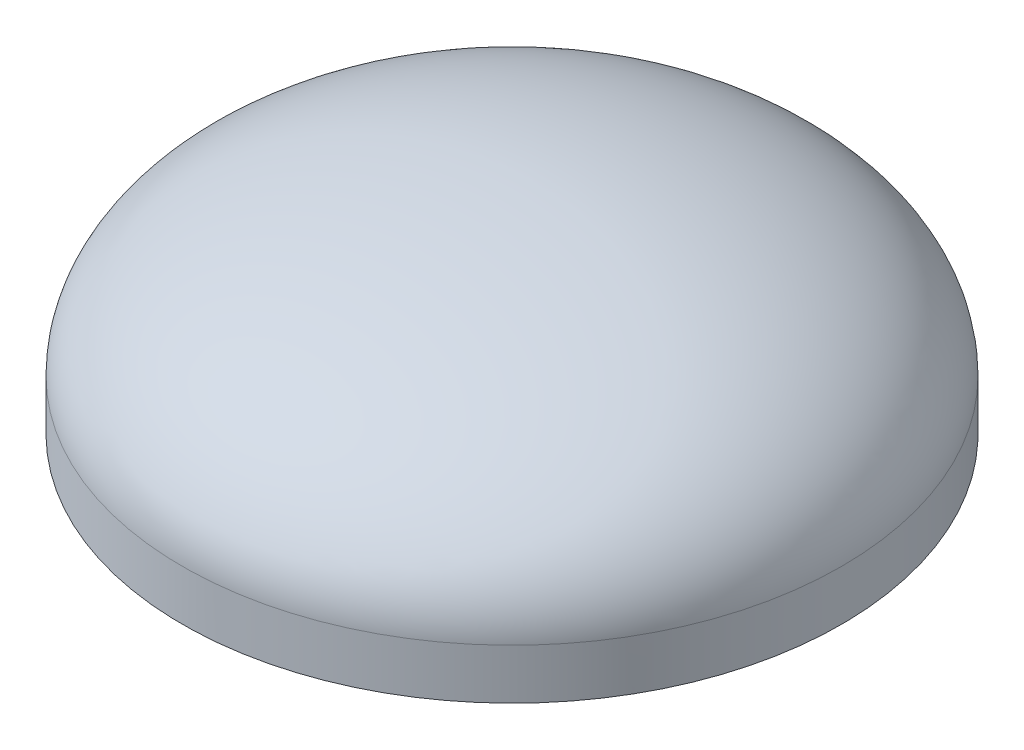
SolidWorks part; units mm, degrees
material "Plain carbon steel"
ref_plane "Front Plane" through (0, 0, 0) normal (0, 0, 1) x (1, 0, 0)
ref_plane "Top Plane" through (0, 0, 0) normal (0, 1, 0) x (1, 0, 0)
ref_plane "Right Plane" through (0, 0, 0) normal (1, 0, 0) x (0, 0, -1)
sketch "Sketch1" plane through (0, 0, 0) normal (0, 0, 1) x (1, 0, 0)
  line L0 (0, 0) -> (162.5, 0) construction
  line L1 (0, 0) -> (0, 106) construction
  point P3 (162.5, 0)
  point P6 (0, 6)
  dimension "DN" = 325
  dimension "H" = 106
  dimension "δ" = 6
sketch "Sketch2" plane through (0, 0, 0) normal (0, 0, 1) x (1, 0, 0)
  line L0 (-162.5, 0) -> (162.5, 0) construction
  line L1 (0, 0) -> (162.5, 0) construction
  line L3 (0, 0) -> (0, 81.25) construction
  line L4 (0, 0) -> (0, -24.75) construction
  line L5 (-162.5, 0) -> (-168.5, 0) construction
  line L6 (0, 81.25) -> (0, 87.25) construction
  line L7 (162.5, 0) -> (168.5, 0) construction
  line L8 (-168.5, 0) -> (-168.5, -24.75)
  line L9 (-168.5, -24.75) -> (-162.5, -24.75)
  line L10 (-162.5, -24.75) -> (-162.5, 0)
  line L11 (0, 81.25) -> (0, 87.25)
  ellipse E0 centre (0, 0) end of major axis (162.5, 0) minor radius 81.25 (0, 81.25) -> (-162.5, 0) ccw
  ellipse E1 centre (0, 0) end of major axis (168.5, 0) minor radius 87.25 (0, 87.25) -> (-168.5, 0) ccw
  dimension "Di" = 325
  dimension "h" = 24.75
  dimension "(H)" = 106
  dimension "δ" = 6
revolve "Revolve1" [suppressed] add sketch "Sketch2" angle 360 mid plane about L3
sketch "Sketch3" plane through (0, 0, 0) normal (0, 0, 1) x (1, 0, 0)
  line L0 (0, 0) -> (0, 81.25) construction
  line L1 (-162.5, 0) -> (162.5, 0) construction
  line L2 (0, 0) -> (162.5, 0) construction
  line L3 (-162.5, -24.75) -> (162.5, -24.75) construction
  line L4 (-162.5, 0) -> (-162.5, -24.75)
  line L5 (-162.5, -24.75) -> (-159.5, -24.75)
  line L6 (-159.5, -24.75) -> (-159.5, 0)
  line L7 (0, 81.25) -> (0, 78.25)
  ellipse E0 centre (0, 0) end of major axis (162.5, 0) minor radius 81.25 (0, 81.25) -> (-162.5, 0) ccw
  ellipse E1 centre (0, 0) end of major axis (159.5, 0) minor radius 78.25 (0, 78.25) -> (-159.5, 0) ccw
  point P3 (0, 78.25)
  point P10 (-159.5, 0)
  point P11 (156.5, 0)
  dimension "D1" = 3
  dimension "δ" = 3
  dimension "(h)" = 24.75
  dimension "D0" = 325
  dimension "D2" = 6
  dimension "H0" = 106
revolve "Revolve2" add sketch "Sketch3" angle 360 mid plane about L0
